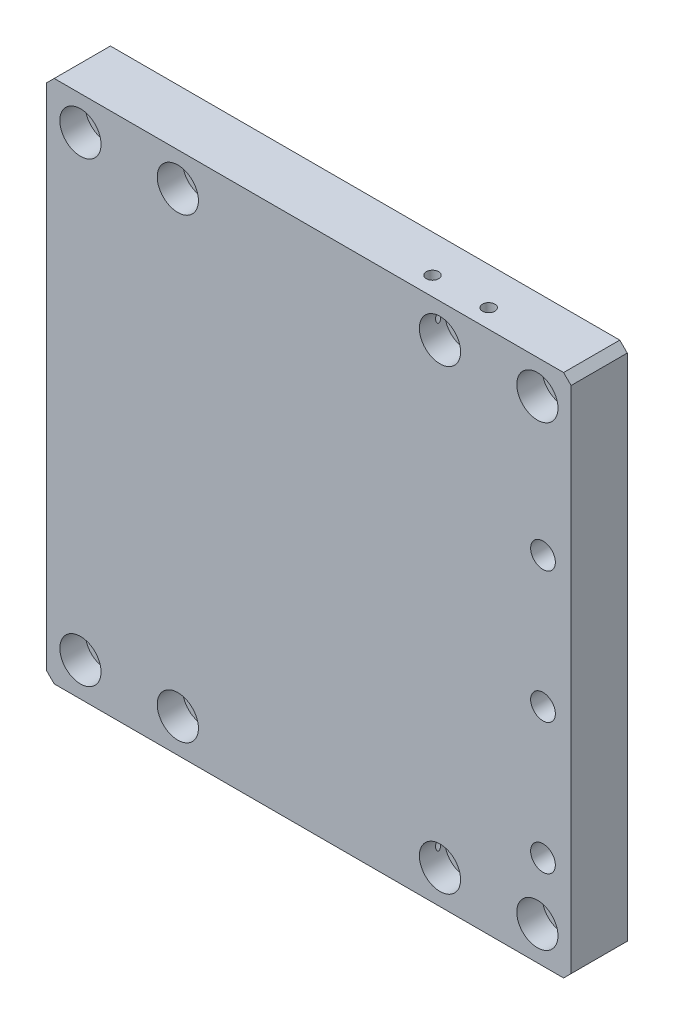
SolidWorks part; units mm, degrees
material "A6061"
ref_plane "前视基准面" through (0, 0, 0) normal (0, 0, 1) x (1, 0, 0)
ref_plane "上视基准面" through (0, 0, 0) normal (0, 1, 0) x (1, 0, 0)
ref_plane "右视基准面" through (0, 0, 0) normal (1, 0, 0) x (0, 0, -1)
sketch "草图1" plane through (0, 0, 0) normal (0, 0, 1) x (1, 0, 0)
  line L1 (-70, -70) -> (70, -70)
  line L2 (-70, -70) -> (-70, 70)
  line L3 (-70, 70) -> (70, 70)
  line L4 (70, -70) -> (70, 70)
  line L5 (-70, -70) -> (70, 70) construction
  line L6 (-70, 70) -> (70, -70) construction
  point P0 (0, 0)
  dimension "D1" = 140
  dimension "D2" = 140
extrude "凸台-拉伸1" add sketch "草图1" along normal blind 15
hole_wizard "打孔尺寸(%根据)内六角圆柱头螺钉的类型1" positions "草图3" profile "草图2" counterbore size "M6" standard "GB"
sketch "草图3" plane through (0, 0, 15) normal (0, 0, 1) x (1, 0, 0)
  line L0 (-70, 61) -> (-61, 61) construction
  line L1 (-70, 70) -> (-70, -70) construction
  line L2 (-61, 61) -> (-35, 61) construction
  line L3 (-35, 61) -> (35, 61) construction
  line L4 (35, 61) -> (61, 61) construction
  line L5 (61, 61) -> (70, 61) construction
  line L6 (70, -70) -> (70, 70) construction
  line L8 (70, 70) -> (-70, 70) construction
  point P0 (-61, 61)
  point P2 (-35, 61)
  point P4 (35, 61)
  point P6 (61, 61)
  dimension "D1" = 26
  dimension "D2" = 9
  dimension "D3" = 70
  dimension "D4" = 9
sketch "草图2" plane through (-61, 61, 15) normal (1, 0, 0) x (0, -1, 0)
  line L0 (0, 0) -> (0, 16.9828)
  line L1 (0, 16.9828) -> (3.3, 15)
  line L2 (3.3, 15) -> (3.3, 6.8)
  line L3 (3.3, 6.8) -> (5.5, 6.8)
  line L4 (5.5, 6.8) -> (5.5, 0)
  line L5 (5.5, 0) -> (0, 0)
  line L10 (0, 16.9828) -> (-3.3, 15) construction
  line L11 (0, -6.35) -> (0, 107.95) construction
  dimension "孔直径" = 6.6
  dimension "孔深度" = 15
  dimension "柱形沉头孔直径" = 11
  dimension "柱形沉头孔深度" = 6.8
  dimension "导头角度" = 118
pattern_linear "阵列(线性)1" count 2 spacing 122 along (0, -1, 0) of "打孔尺寸(%根据)内六角圆柱头螺钉的类型1"
hole_wizard "打孔尺寸(%根据)内六角圆柱头螺钉的类型2" positions "草图5" profile "草图6" counterbore size "M6" standard "GB" end condition through all
sketch "草图5" plane through (0, 0, 0) normal (0, 0, -1) x (-1, 0, 0)
  point P0 (-62.5, 25)
  point P3 (-62.5, -10)
  point P6 (-62.5, -45)
sketch "草图6" plane through (62.5, 25, 0) normal (1, 0, 0) x (0, 1, 0)
  line L0 (0, 0) -> (0, 15)
  line L1 (0, 15) -> (3.3, 15)
  line L3 (3.3, 15) -> (3.3, 6.8)
  line L4 (3.3, 6.8) -> (5.5, 6.8)
  line L5 (5.5, 6.8) -> (5.5, 0)
  line L7 (5.5, 0) -> (0, 0)
  line L11 (0, -6.35) -> (0, 107.95) construction
  dimension "通孔孔直径" = 6.6
  dimension "通孔孔深度" = 15
  dimension "柱形沉头孔直径" = 11
  dimension "柱形沉头孔深度" = 6.8
hole_wizard "M4 螺纹孔1" positions "草图8" profile "草图7" tap size "M4" standard "GB"
sketch "草图8" plane through (0, 70, 0) normal (0, 1, 0) x (1, 0, 0)
  line L0 (28, -10) -> (43, -10) construction
  line L1 (43, -10) -> (70, -10) construction
  line L2 (70, -15) -> (70, 0) construction
  line L4 (70, -15) -> (-70, -15) construction
  point P0 (28, -10)
  point P2 (43, -10)
  dimension "D1" = 27
  dimension "D2" = 15
  dimension "D3" = 5
cosmetic thread "孔螺蚊线1" parameters "D1"=12, "D2"=4
cosmetic thread "孔螺蚊线2" parameters "D1"=12, "D2"=4
sketch "草图7" plane through (28, 70, 10) normal (1, 0, 0) x (0, 0, 1)
  line L0 (0, 0) -> (0, 15.0914)
  line L1 (0, 15.0914) -> (1.65, 14.1)
  line L2 (1.65, 14.1) -> (1.65, 0)
  line L5 (1.65, 0) -> (0, 0)
  line L10 (0, 15.0914) -> (-1.65, 14.1) construction
  line L11 (0, -6.35) -> (0, 107.95) construction
  dimension "螺纹孔钻头直径" = 3.3
  dimension "螺纹孔钻头深度" = 14.1
  dimension "导头角度" = 118
chamfer "倒角1" distance 2 angle 45 4 edges at (-70, -70, 7.5) (70, -70, 7.5) (70, 70, 7.5) (-70, 70, 7.5)
mirror "镜向1" about plane through (0, 0, 0) normal (0, 1, 0) of "M4 螺纹孔1"
